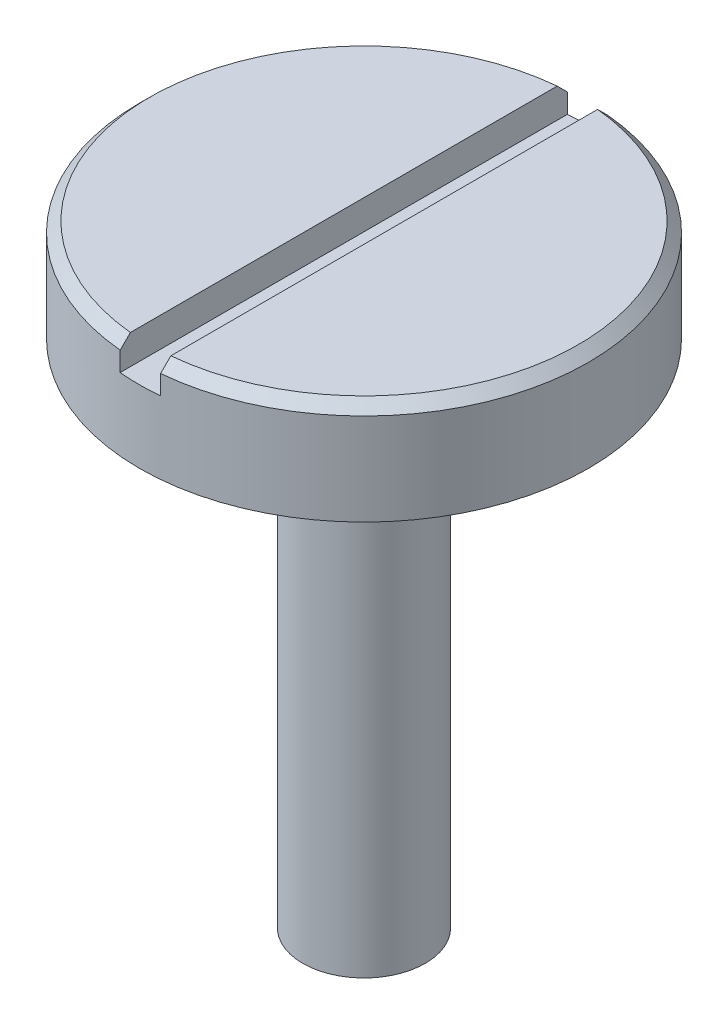
SolidWorks part; units mm, degrees
ref_plane "Front Plane" through (0, 0, 0) normal (0, 0, 1) x (1, 0, 0)
ref_plane "Top Plane" through (0, 0, 0) normal (0, 1, 0) x (1, 0, 0)
ref_plane "Right Plane" through (0, 0, 0) normal (1, 0, 0) x (0, 0, -1)
sketch "Sketch1" plane through (0, 0, 0) normal (0, 0, 1) x (1, 0, 0)
  line L0 (0, 28.3508) -> (0, -18.7556) construction
  line L1 (0, 21.2019) -> (-11, 21.2019)
  line L2 (-11, 21.2019) -> (-11, 16.2019)
  line L3 (-11, 16.2019) -> (-3, 16.2019)
  line L4 (-3, 16.2019) -> (-3, -8.7981)
  line L5 (-3, -8.7981) -> (0, -8.7981)
  line L6 (0, -8.7981) -> (0, 21.2019)
  dimension "D1" = 30
  dimension "D2" = 5
  dimension "D3" = 3
  dimension "D4" = 11
revolve "Revolve1" add sketch "Sketch1" angle 360 about L0
sketch "Sketch2" plane through (0, 0, 0) normal (0, 0, 1) x (1, 0, 0)
  line L0 (11, 21.2019) -> (-11, 21.2019) construction
  line L1 (-0.99, 22.6517) -> (0.99, 22.6517)
  line L2 (-0.99, 22.6517) -> (-0.99, 19.752)
  line L3 (-0.99, 19.752) -> (0.99, 19.752)
  line L4 (0.99, 22.6517) -> (0.99, 19.752)
  line L5 (-0.99, 22.6517) -> (0.99, 19.752) construction
  line L6 (-0.99, 19.752) -> (0.99, 22.6517) construction
  point P0 (0, 21.2019)
extrude "Cut-Extrude1" cut sketch "Sketch2" against normal mid plane 36
chamfer "Chamfer1" distance 0.5 angle 45 2 edges at (11, 21.2019, 0) (-11, 21.2019, 0)
